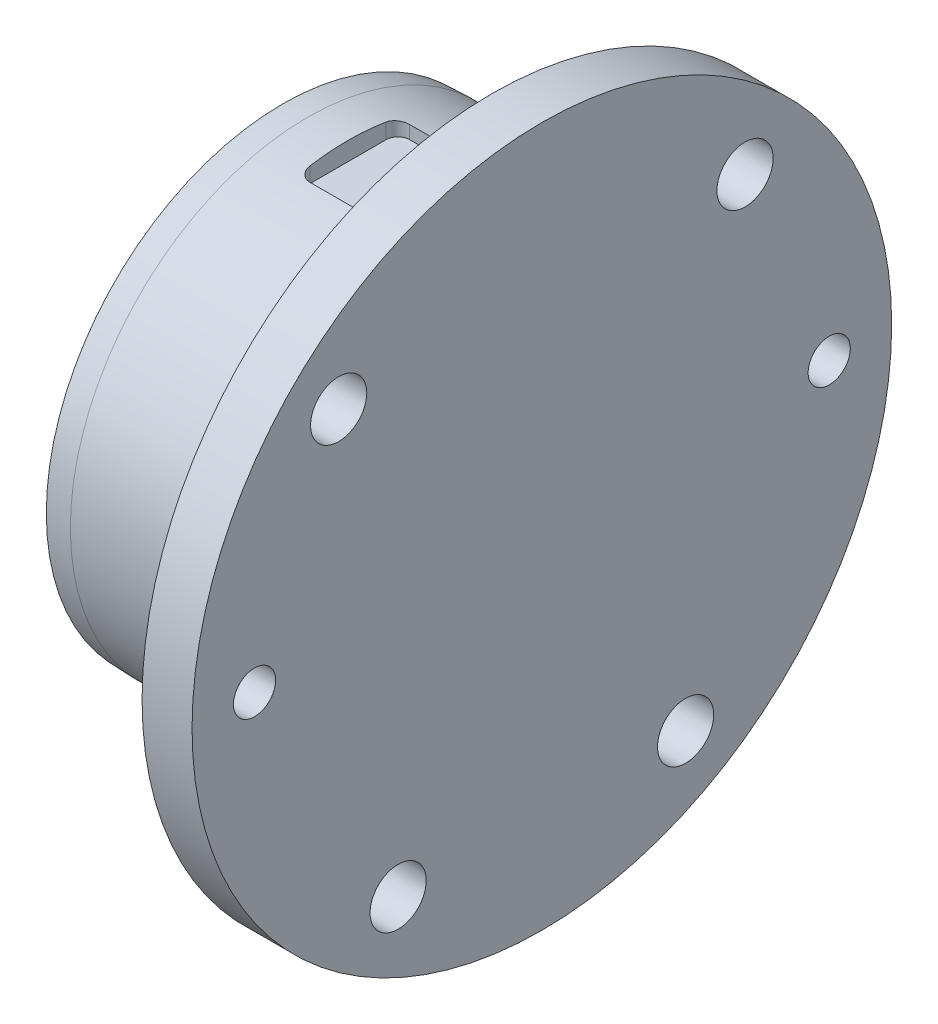
from build123d import *

# Parameters (mm, degrees)
F_9_16_0_5625_DIAMETER_HOLE1_D = 14.2875
F_1_2_13_TAPPED_HOLE1_D        = 10.71626
EXTRUDE1_START                 = 55.626
SKETCH8_W                      = 36.576
SKETCH8_H                      = 25.4
EXTRUDE1_DEPTH                 = 4.6863
EXTRUDE2_REACH                 = 184.013
EXTRUDE2_END_RADIUS            = 46.865
FILLET1_R                      = 3


with BuildPart() as part:
    # Sketch1 → Revolve1 (revolve)
    with BuildSketch(Plane.XY):
        Polygon((-65.8622, 50.618781854), (-65.8622, 60.0705), (-59.5122, 60.3123), (-12.7, 60.3123), (-12.7, 88.9), (0, 88.9), (0, 0), (-18.159, 0), (-18.159, 46.865), (-33.909, 46.865), (-33.909, 50.00625), (-58.7756, 50.00625), (-58.7756, 53.0098), (-61.8236, 53.0098), (-61.8236, 50.00625), (-63.5762, 50.00625), align=None)
    revolve(axis=Axis((0, 0, 0), (-1, 0, 0)))

    # 9/16 (0.5625) Diameter Hole1 (through all)
    with Locations(Plane(origin=(0, 0, 0), x_dir=(0, 0, -1), z_dir=(1, 0, 0))):
        with Locations((-51.6382, 51.6382), (51.6382, 51.6382), (-36.5252, -63.246), (36.5252, -63.246)):
            Hole(F_9_16_0_5625_DIAMETER_HOLE1_D / 2)

    # 1/2-13 Tapped Hole1 (through all)
    with Locations(Plane(origin=(0, 0, 0), x_dir=(0, 0, -1), z_dir=(1, 0, 0))):
        with Locations((-73.025, 0), (73.025, 0)):
            Hole(F_1_2_13_TAPPED_HOLE1_D / 2)

    # Sketch8 → Extrude1 (cut)
    with BuildSketch(Plane(origin=(0, 0, 0), x_dir=(1, 0, 0), z_dir=(0, 1, 0)).offset(EXTRUDE1_START)):
        with Locations((-30.988, 0)):
            Rectangle(SKETCH8_W, SKETCH8_H)
    extrude(amount=EXTRUDE1_DEPTH, mode=Mode.SUBTRACT)

    # Extrude2: up to this cylinder (the profile starts outside it)
    extrude2_end = Plane(origin=(-18.090047, 0, 0), z_dir=(1, 0, 0)) * Cylinder(EXTRUDE2_END_RADIUS, 462.756, mode=Mode.PRIVATE)
    # Sketch9 → Extrude2 (cut, up to the surface)
    with BuildSketch(Plane(origin=(0, 55.626, 0), x_dir=(1, 0, 0), z_dir=(0, 1, 0)), mode=Mode.PRIVATE) as extrude2_sk1:
        with BuildLine():
            Line((-12.7, 12.7), (-12.7, -12.7))
            ThreePointArc((-12.7, -12.7), (-25.4, 0), (-12.7, 12.7))
        make_face()
    extrude2_tool1 = extrude(extrude2_sk1.sketch, amount=-EXTRUDE2_REACH, mode=Mode.PRIVATE) - extrude2_end
    add(extrude2_tool1.solids().sort_by_distance((-18.090047, 55.626, 0))[0], mode=Mode.SUBTRACT)

    # Fillet1
    fillet1_edges = [part.edges().sort_by_distance(p)[0] for p in [
        (-49.276, 57.293008189, 12.7),
        (-49.276, 57.293008189, -12.7),
    ]]
    fillet(fillet1_edges, radius=FILLET1_R)


solid = part.part
